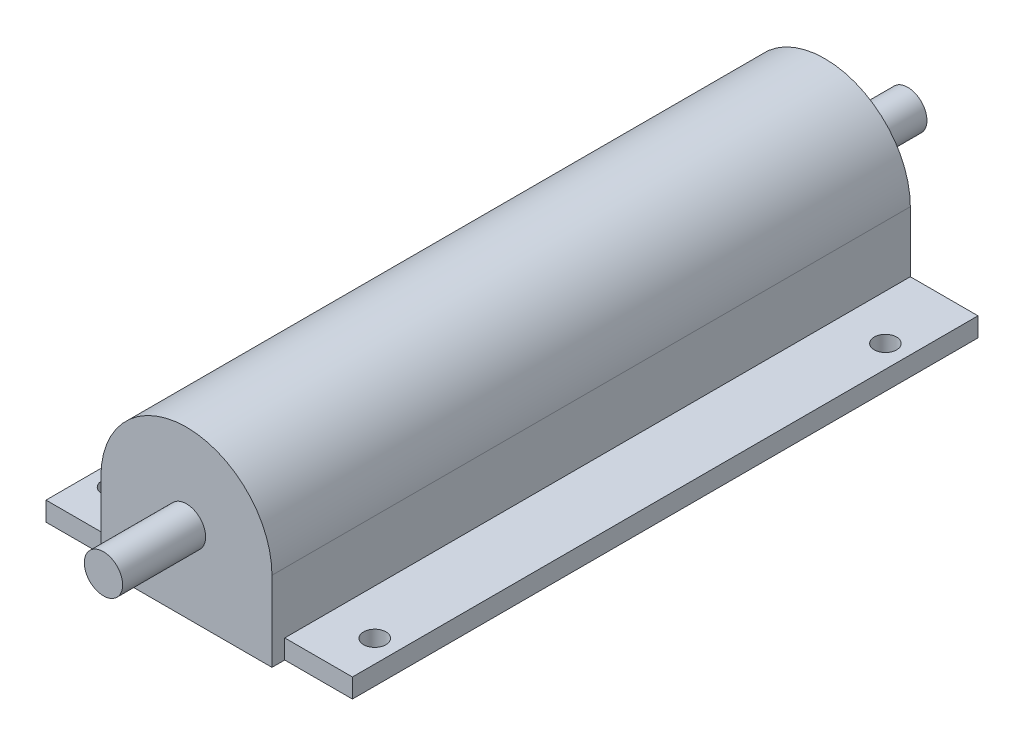
from build123d import *

# Parameters (mm, degrees)
EXTRUDE_1_DEPTH     = 100
SKETCH_2_W          = 98
SKETCH_2_H          = 3
EXTRUDE_2_DEPTH     = 10.6
SKETCH_3_W          = 2
SKETCH_3_H          = 6.4
CUT_EXTRUDE_1_DEPTH = 107.050978308
SKETCH_4_W          = 98
SKETCH_4_H          = 4.9
EXTRUDE_3_DEPTH     = 12.6
SKETCH_5_W          = 10.6
SKETCH_5_H          = 1.9
CUT_EXTRUDE_2_DEPTH = 107.050978308
SKETCH_6_R          = 3
EXTRUDE_4_DEPTH     = 13
EXTRUDE_START       = 13
SKETCH_7_R          = 3
EXTRUDE_5_DEPTH     = 13
SKETCH_10_R         = 1.75
CUT_EXTRUDE_3_DEPTH = 10


with BuildPart() as part:
    # 草图1 → 凸台-拉伸1 (new body)
    with BuildSketch(Plane.XY.offset(49)):
        with BuildLine():
            Line((-13.4, 0), (13.4, 0))
            Line((13.4, 0), (13.4, 12.5))
            ThreePointArc((13.4, 12.5), (0, 25.9), (-13.4, 12.5))
            Line((-13.4, 12.5), (-13.4, 0))
        make_face()
    extrude(amount=-EXTRUDE_1_DEPTH)

    # 草图2 → 凸台-拉伸2 (add)
    with BuildSketch(Plane(origin=(13.4, 0, 0), x_dir=(0, 0, -1), z_dir=(1, 0, 0))):
        with Locations((2, 1.5)):
            Rectangle(SKETCH_2_W, SKETCH_2_H)
    extrude(amount=EXTRUDE_2_DEPTH)

    # 草图3 → 切除-拉伸1 (cut, through all)
    with BuildSketch(Plane.XY.offset(49)):
        with Locations((-12.4, -0.2)):
            Rectangle(SKETCH_3_W, SKETCH_3_H)
    extrude(amount=-CUT_EXTRUDE_1_DEPTH, mode=Mode.SUBTRACT)

    # 草图4 → 凸台-拉伸3 (add)
    with BuildSketch(Plane.ZY.offset(11.4)):
        with Locations((-2, 2.45)):
            Rectangle(SKETCH_4_W, SKETCH_4_H)
    extrude(amount=EXTRUDE_3_DEPTH)

    # 草图5 → 切除-拉伸2 (cut, through all)
    with BuildSketch(Plane(origin=(0, 0, -51), x_dir=(-1, 0, 0), z_dir=(0, 0, -1))):
        with Locations((18.7, 3.95)):
            Rectangle(SKETCH_5_W, SKETCH_5_H)
    extrude(amount=-CUT_EXTRUDE_2_DEPTH, mode=Mode.SUBTRACT)

    # 草图6 → 凸台-拉伸4 (add)
    with BuildSketch(Plane.XY.offset(49)):
        with Locations(Location((0, 12.5, 0), (0, 0, 180))):
            Circle(SKETCH_6_R)
    extrude(amount=EXTRUDE_4_DEPTH)

    # 草图7 → 凸台-拉伸5 (add)
    with BuildSketch(Plane(origin=(0, 0, -51), x_dir=(-1, 0, 0), z_dir=(0, 0, -1)).offset(EXTRUDE_START)):
        with Locations((0, 12.5)):
            Circle(SKETCH_7_R)
    extrude(amount=-EXTRUDE_5_DEPTH)

    # 草图10 → 切除-拉伸3 (cut)
    with BuildSketch(Plane.XZ):
        with Locations(Location((-20.5, 40, 0), (0, 0, 270))):
            Circle(SKETCH_10_R)
        with Locations(Location((20.5, 40, 0), (0, 0, 270))):
            Circle(SKETCH_10_R)
        with Locations(Location((20.5, -40, 0), (0, 0, 270))):
            Circle(SKETCH_10_R)
        with Locations(Location((-20.5, -40, 0), (0, 0, 270))):
            Circle(SKETCH_10_R)
    extrude(amount=-CUT_EXTRUDE_3_DEPTH, mode=Mode.SUBTRACT)


solid = part.part
